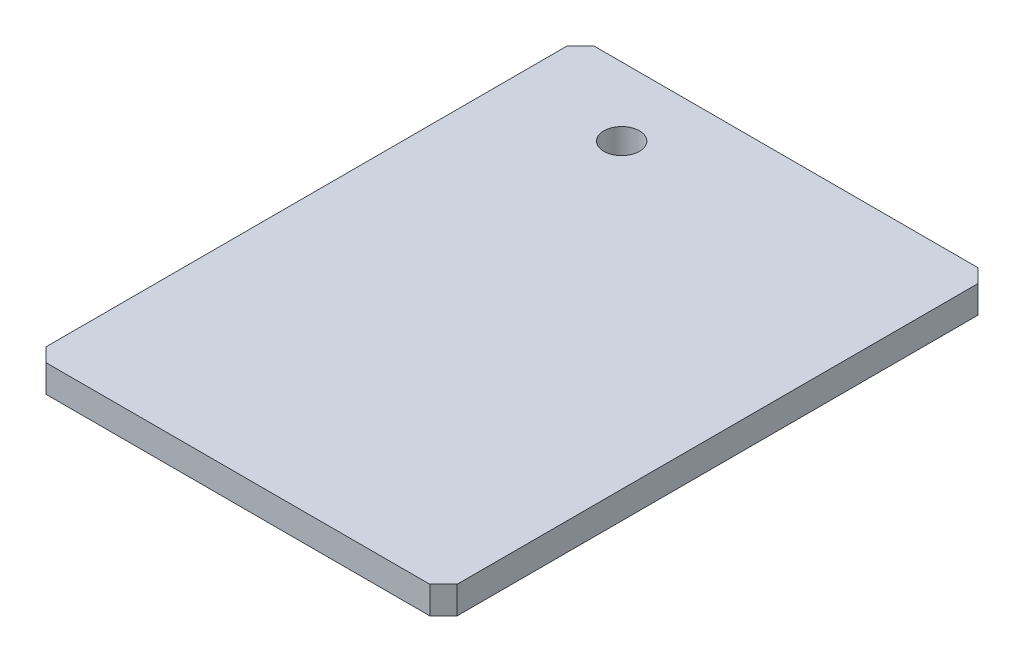
from build123d import *

# Parameters (mm, degrees)
SKETCH_1_W          = 300
SKETCH_1_H          = 400
EXTRUDE_1_DEPTH     = 20
CHAMFER_1_SIZE      = 10
HOLE_WIZARD_M24_1_D = 26


with BuildPart() as part:
    # 草图1 → 凸台-拉伸1 (new body)
    with BuildSketch(Plane(origin=(0, 0, 0), x_dir=(1, 0, 0), z_dir=(0, 1, 0))):
        Rectangle(SKETCH_1_W, SKETCH_1_H)
    extrude(amount=EXTRUDE_1_DEPTH)

    # 倒角1
    chamfer_1_edges = [part.edges().sort_by_distance(p)[0] for p in [
        (150, 10, 200),
        (-150, 10, 200),
        (-150, 10, -200),
        (150, 10, -200),
    ]]
    chamfer(chamfer_1_edges, length=CHAMFER_1_SIZE)

    # M24 间隙孔1 (through all)
    with Locations(Plane(origin=(0, 0, 0), x_dir=(-1, 0, 0), z_dir=(0, -1, 0))):
        with Locations((70, 150)):
            Hole(HOLE_WIZARD_M24_1_D / 2)


solid = part.part
